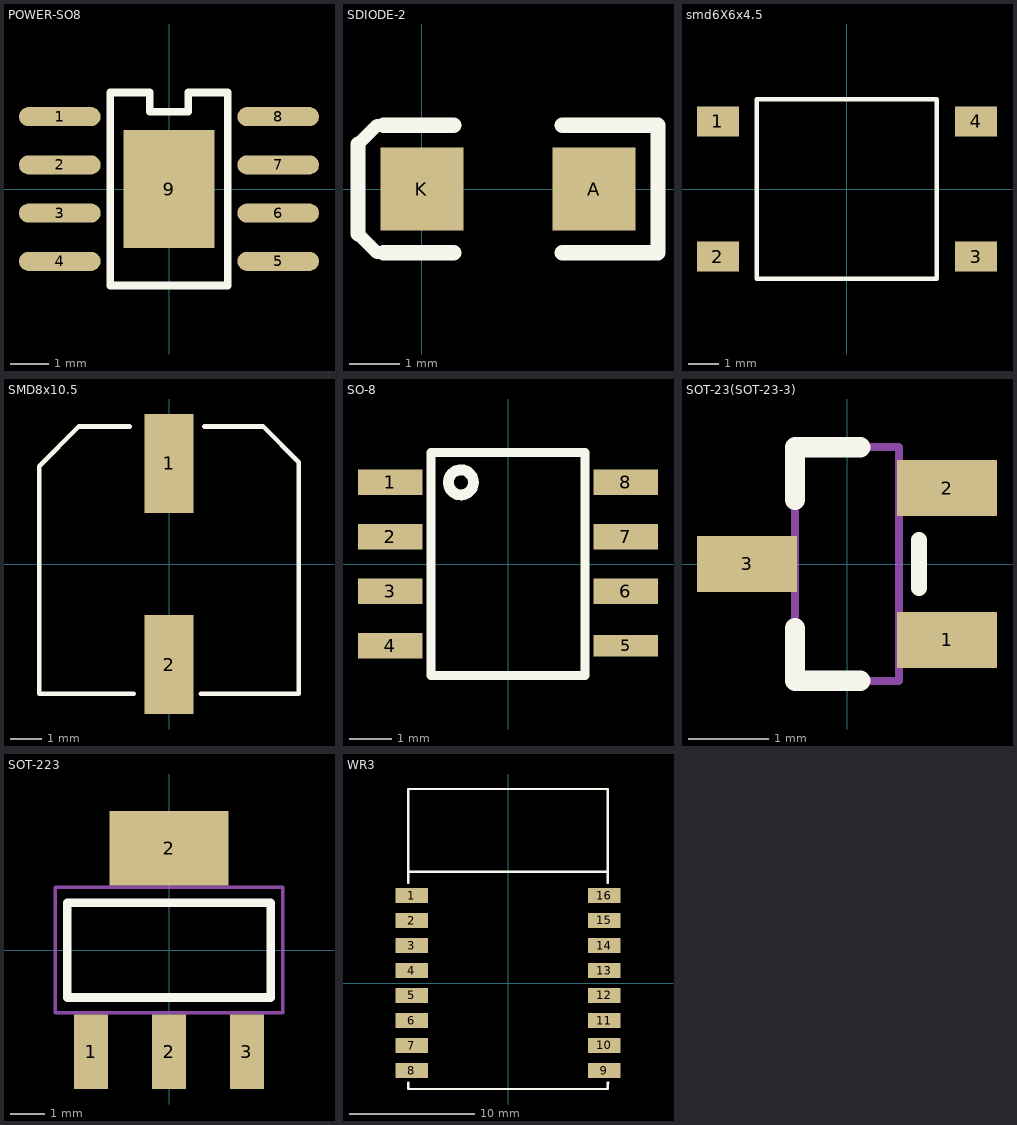
[diagram p0: the footprints below, top view; thin cyan lines are the x and y axes]
# Altium footprint library MISC82282.PcbLib: 24 footprints (part 2 of 2)
Each footprint in its own frame and in the unit in brackets; x right, y up, seen from the top. Pads: shape width x height; smd on the part's side, far side on the other; paste and mask are expansions set on the pad; w line width, h text height; cw(c..) or ccw(c..) is an arc to the next point about the centre after c.

## POWER-SO8 [mm]
pads (9):
  oval 2.15x0.5 smd: 1(-2.875,1.905) 2(-2.875,0.635) 3(-2.875,-0.635) 4(-2.875,-1.905) 5(2.875,-1.905) 6(2.875,-0.635) 7(2.875,0.635) 8(2.875,1.905)
  rect 2.4x3.1 smd: 9(0,0)
Top Overlay:
  lines w0.2: -1.55,-2.54 -1.55,2.54 -0.508,2.54 -0.508,2.032 0.508,2.032 0.508,2.54 1.55,2.54 1.55,-2.54 -1.55,-2.54

## SDIODE-2 [mil]
height 156.69
pads (2):
  rect 65x65 smd: A(135,0) K(0,0)
Top Overlay:
  lines w10: -50,-35 -35,-50 -30,-50 ; -50,35 -35,50 -30,50
  lines w12: -50,-35 -50,35 ; -30,-50 25,-50 ; -30,50 25,50 ; 110,-50 185,-50 185,50 110,50

## smd6X6x4.5 [mm]
pads (4):
  rect 1.4x1 smd: 1(-4.3,2.25) 2(-4.3,-2.25) 3(4.3,-2.25) 4(4.3,2.25)
Top Overlay:
  lines w0.15: -3,-3 -3,3 3,3 3,-3 -3,-3

## SMD8x10.5 [mm]
pads (2):
  rect 1.6x3.2 smd: 1(0,3.25) 2(0,-3.25)
Top Overlay:
  lines w0.15: -1.27,4.445 -2.921,4.445 -4.2,3.166 -4.2,2.6 -4.2,-4.2 -1.143,-4.2 ; 1.025,-4.2 4.2,-4.2 4.2,2.6 4.2,3.293 3.048,4.445 1.143,4.445

## SO-8 [mm]
pads (8):
  rect 1.5x0.6 smd: 1(-2.75,1.905) 2(-2.75,0.635) 3(-2.75,-0.635) 4(-2.75,-1.905) 6(2.75,-0.635) 7(2.75,0.635) 8(2.75,1.905)
  rect 1.5x0.5 smd: 5(2.75,-1.905)
Top Overlay:
  circle w0.254: c-1.099,1.905 r0.292
  lines w0.203: 1.796,2.603 -1.797,2.603 -1.797,-2.603 1.797,-2.603 1.797,2.604

## SOT-23(SOT-23-3) [mm]
height 3.98
pads (3):
  rect 1.25x0.7 smd: 1(1.25,-0.95) 2(1.25,0.95) 3(-1.25,0)
Top Overlay:
  lines w0.2: 0.9,-0.3 0.9,0.3
  lines w0.254: -0.65,-0.8 -0.65,-1.46 0.165,-1.46 ; 0.165,1.46 -0.65,1.46 ; -0.65,0.8 -0.65,1.46 ; -0.65,0.8 -0.65,1.46 ; -0.65,0.8 -0.65,1.46
Mechanical 13:
  lines w0.1: -0.65,-1.46 -0.65,1.46 ; -0.65,-1.46 0.65,-1.46 ; -0.65,-1.46 -0.65,1.46 ; -0.65,-1.46 0.65,-1.46 ; -0.65,-1.46 0.65,-1.46 ; -0.65,-1.46 -0.65,1.46 ; -0.65,1.46 0.65,1.46 ; -0.65,1.46 0.65,1.46 ; -0.65,1.46 0.65,1.46 ; 0.65,-1.46 0.65,1.46 ; 0.65,-1.46 0.65,1.46 ; 0.65,-1.46 0.65,1.46
3D body: height 1.3, standoff 0, extent -1.5,-1.5 1.5,1.5

## SOT-223 [mm]
pads (4):
  rect 1x2.2 smd: 1(-2.3,-3) 2(0,-3) 3(2.3,-3)
  rect 3.5x2.2 smd: 2(0,3)
Top Overlay:
  lines w0.254: -3,-1.4 -3,1.4 3,1.4 3,-1.4 -3,-1.4
Mechanical 13:
  lines w0.1: -3.35,-1.85 -3.35,1.85 3.35,1.85 3.35,-1.85 -3.35,-1.85
3D body: height 1.64, standoff -0.04, extent -3.242,-3.49 3.243,3.49

## WR3 [mm]
height 3.98
pads (16):
  rect 2.6x1.2 smd: 1(-7.7,7) 2(-7.7,5) 3(-7.7,3) 4(-7.7,1) 5(-7.7,-1) 6(-7.7,-3) 7(-7.7,-5) 8(-7.7,-7) 9(7.7,-7) 10(7.7,-5) 11(7.7,-3) 12(7.7,-1) 13(7.7,1) 14(7.7,3) 15(7.7,5) 16(7.7,7)
Top Overlay:
  lines w0.2: -8,-7.975 -8,-8.48 8,-8.48 8,-7.977 8.002,-7.975 ; -8,8.027 -8,15.52 8,15.52 8,8.029 ; -8,8.89 8,8.89